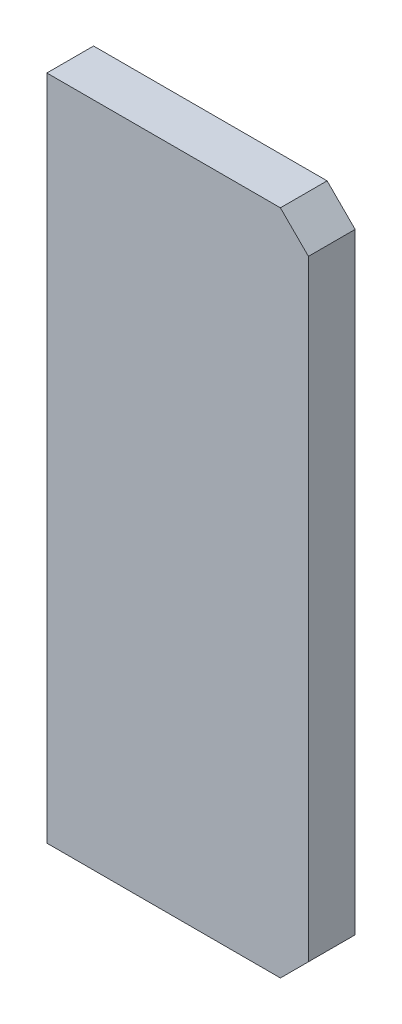
SolidWorks part; units mm, degrees
material "Q235"
ref_plane "Front Plane" through (0, 0, 0) normal (0, 0, 1) x (1, 0, 0)
ref_plane "Top Plane" through (0, 0, 0) normal (0, 1, 0) x (1, 0, 0)
ref_plane "Right Plane" through (0, 0, 0) normal (1, 0, 0) x (0, 0, -1)
sketch "Sketch1" plane through (0, 0, 0) normal (0, 0, 1) x (1, 0, 0)
  line L1 (0, 0) -> (140, 0)
  line L2 (0, 0) -> (0, 357)
  line L3 (0, 357) -> (140, 357)
  line L4 (140, 0) -> (140, 357)
  dimension "D1" = 140
  dimension "D2" = 357
extrude "Boss-Extrude1" add sketch "Sketch1" along normal blind 25
chamfer "Chamfer2" distance 15 angle 45 2 edges at (140, 0, 12.5) (140, 357, 12.5)
